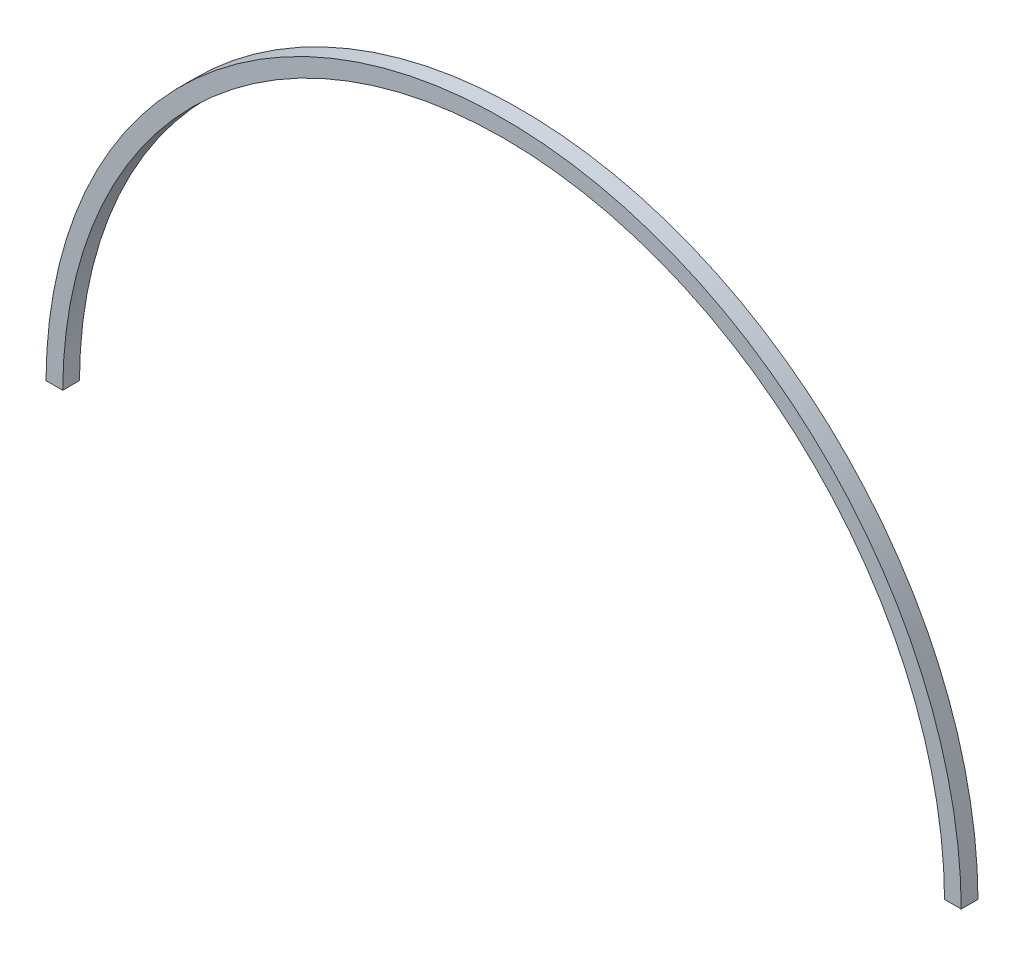
SolidWorks part; units mm, degrees
ref_plane "前视基准面" through (0, 0, 0) normal (0, 0, 1) x (1, 0, 0)
ref_plane "上视基准面" through (0, 0, 0) normal (0, 1, 0) x (1, 0, 0)
ref_plane "右视基准面" through (0, 0, 0) normal (1, 0, 0) x (0, 0, -1)
other "Configuration Table"
sketch "草图1" plane through (0, 0, 0) normal (0, 0, 1) x (1, 0, 0)
  line L0 (1.0023, 1) -> (9.0024, 1)
  line L1 (430.9976, 1) -> (438.9977, 1)
  arc A0 (438.9977, 1) -> (1.0023, 1) centre (220, 0) ccw
  arc A1 (9.0024, 1) -> (430.9976, 1) centre (220, 0) cw
  point P0 (0, 0)
  dimension "D1" = 219
  dimension "D2" = 211
  dimension "D3" = 8.0001
  dimension "D4" = 438.9977
extrude "凸台-拉伸1" add sketch "草图1" against normal mid plane 8
